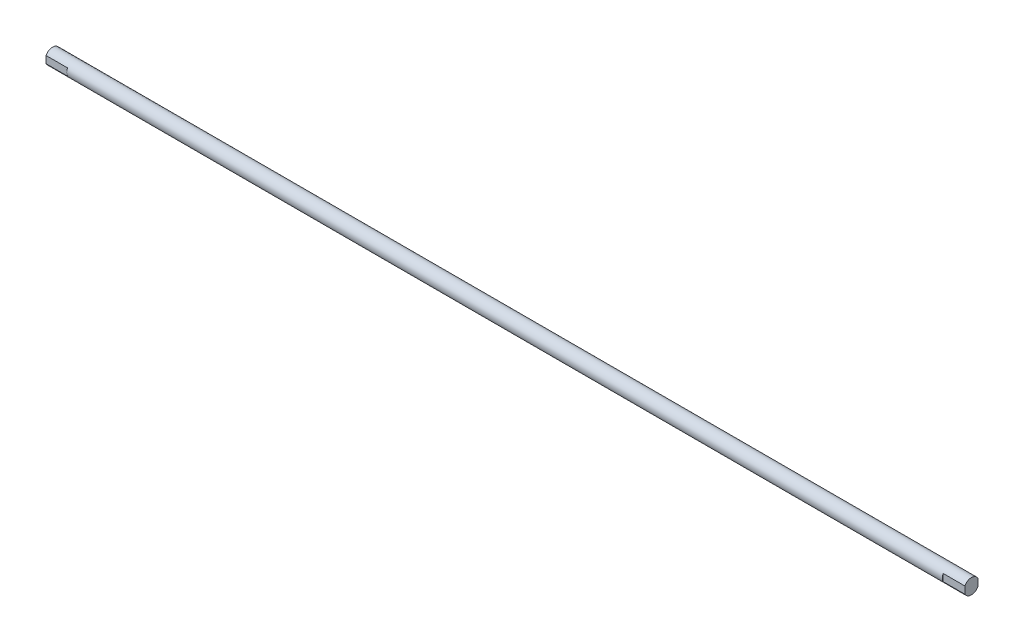
from build123d import *

# Parameters (mm, degrees)
SKETCH1_R           = 12.5
BOSS_EXTRUDE1_DEPTH = 1530
CUT_EXTRUDE1_START  = -11
SKETCH_2_2_W        = 44.374102045
SKETCH_2_2_H        = 48.77153558
SKETCH_2_2_W_2      = 134.556182266
SKETCH_2_2_H_2      = 57.966169337
CUT_EXTRUDE1_DEPTH  = 20
CUT_EXTRUDE2_START  = 11
SKETCH_2_2_2_W      = 44.374102045
SKETCH_2_2_2_H      = 48.77153558
SKETCH_2_2_2_W_2    = 134.556182266
SKETCH_2_2_2_H_2    = 57.966169337
CUT_EXTRUDE2_DEPTH  = 20


with BuildPart() as part:
    # Sketch1 → Boss-Extrude1 (new body)
    with BuildSketch(Plane(origin=(0, 0, 0), x_dir=(0, 0, -1), z_dir=(1, 0, 0))):
        Circle(SKETCH1_R)
    extrude(amount=BOSS_EXTRUDE1_DEPTH)

    # Sketch 2_2 → Cut-Extrude1 (cut)
    with BuildSketch(Plane.XY.offset(CUT_EXTRUDE1_START)):
        with Locations((13.812948977, 5.596733591)):
            Rectangle(SKETCH_2_2_W, SKETCH_2_2_H)
        with Locations((1561.278091133, 0.999416713)):
            Rectangle(SKETCH_2_2_W_2, SKETCH_2_2_H_2)
    extrude(amount=-CUT_EXTRUDE1_DEPTH, mode=Mode.SUBTRACT)

    # Sketch 2_2 2 → Cut-Extrude2 (cut)
    with BuildSketch(Plane.XY.offset(CUT_EXTRUDE2_START)):
        with Locations((13.812948977, 5.596733591)):
            Rectangle(SKETCH_2_2_2_W, SKETCH_2_2_2_H)
        with Locations((1561.278091133, 0.999416713)):
            Rectangle(SKETCH_2_2_2_W_2, SKETCH_2_2_2_H_2)
    extrude(amount=CUT_EXTRUDE2_DEPTH, mode=Mode.SUBTRACT)


solid = part.part
